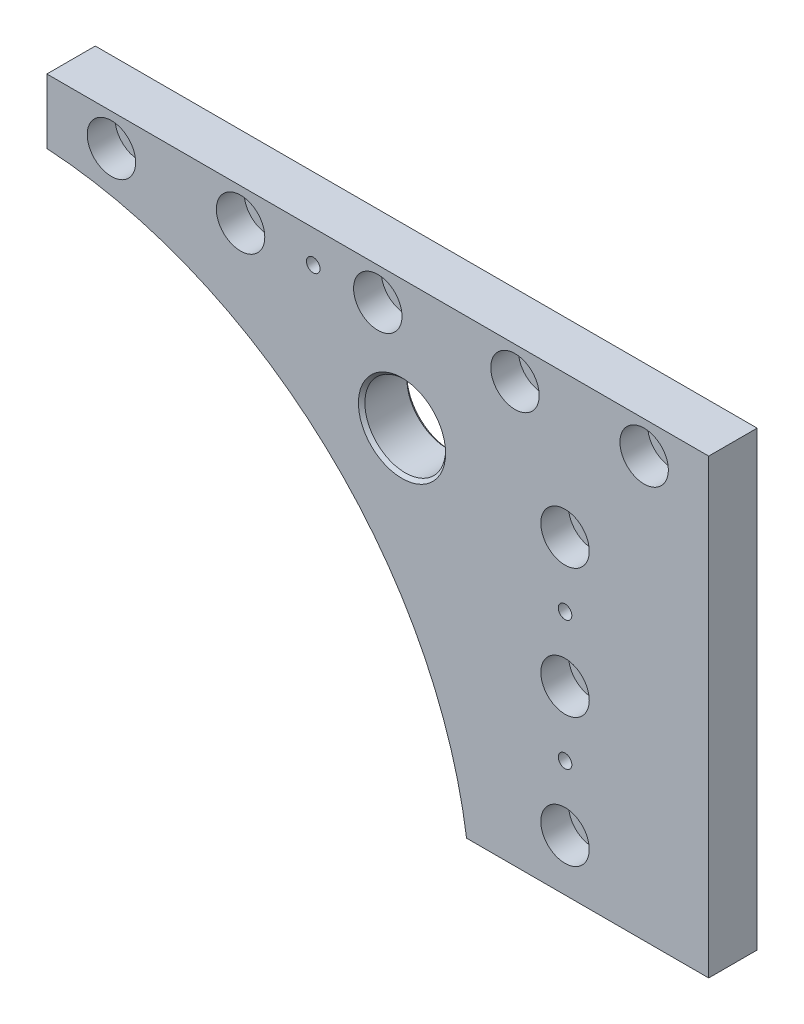
from build123d import *

# Parameters (mm, degrees)
EXTRUDE_1_DEPTH              = 7.5
HOLE_WIZARD_M8_2_D           = 9
HOLE_WIZARD_M8_2_CBORE_D     = 15
HOLE_WIZARD_M8_2_CBORE_DEPTH = 8.6
HOLE_WIZARD_M5_1_D           = 4.2
HOLE_WIZARD_M5_1_DEPTH       = 12.4
HOLE_WIZARD_M5_1_TIP         = 1.2618073
SKETCH_11_R                  = 140
CUT_EXTRUDE_2_DEPTH          = 249.696602309
SKETCH_12_R                  = 12.5
CUT_EXTRUDE_3_DEPTH          = 326.153809758
CHAMFER_1_SIZE               = 1


with BuildPart() as part:
    # 草图1 → 凸台-拉伸1 (new, symmetric)
    with BuildSketch(Plane.XY):
        Polygon((0, 0), (205, 0), (205, -140), (130, -140), (0, -20), align=None)
    extrude(amount=EXTRUDE_1_DEPTH, both=True)

    # M8 六角凹头螺钉的柱形沉头孔2 (through all)
    with Locations(Plane.XY.offset(7.5)):
        with Locations((20, -10), (60, -10), (145, -10), (102.5, -10), (185, -10), (160.5, -44), (160.5, -84), (160.5, -124)):
            CounterBoreHole(HOLE_WIZARD_M8_2_D / 2, HOLE_WIZARD_M8_2_CBORE_D / 2, HOLE_WIZARD_M8_2_CBORE_DEPTH)

    # M5 螺纹孔1
    with Locations(Plane.XY.offset(7.5)):
        with Locations((82.5, -10), (143.75, -10), (160.5, -64), (160.5, -104)):
            Hole(HOLE_WIZARD_M5_1_D / 2, depth=HOLE_WIZARD_M5_1_DEPTH)
            with Locations((0, 0, -(HOLE_WIZARD_M5_1_DEPTH + HOLE_WIZARD_M5_1_TIP / 2))):  # 118° drill point
                Cone(0, HOLE_WIZARD_M5_1_D / 2, HOLE_WIZARD_M5_1_TIP, mode=Mode.SUBTRACT)

    # 草图11 → 切除-拉伸2 (cut, through all)
    with BuildSketch(Plane.XY.offset(7.5)):
        with Locations((-8.60198636, -159.735485224)):
            Circle(SKETCH_11_R)
    extrude(amount=-CUT_EXTRUDE_2_DEPTH, mode=Mode.SUBTRACT)

    # 草图12 → 切除-拉伸3 (cut, through all)
    with BuildSketch(Plane(origin=(0, 0, -202.5), x_dir=(-1, 0, 0), z_dir=(0, 0, -1))):
        with Locations((-110, -40)):
            Circle(SKETCH_12_R)
    extrude(amount=-CUT_EXTRUDE_3_DEPTH, mode=Mode.SUBTRACT)

    # 倒角1
    chamfer_1_edges = [part.edges().sort_by_distance(p)[0] for p in [
        (122.5, -40, 7.5),
        (122.5, -40, -7.5),
    ]]
    chamfer(chamfer_1_edges, length=CHAMFER_1_SIZE)


solid = part.part
